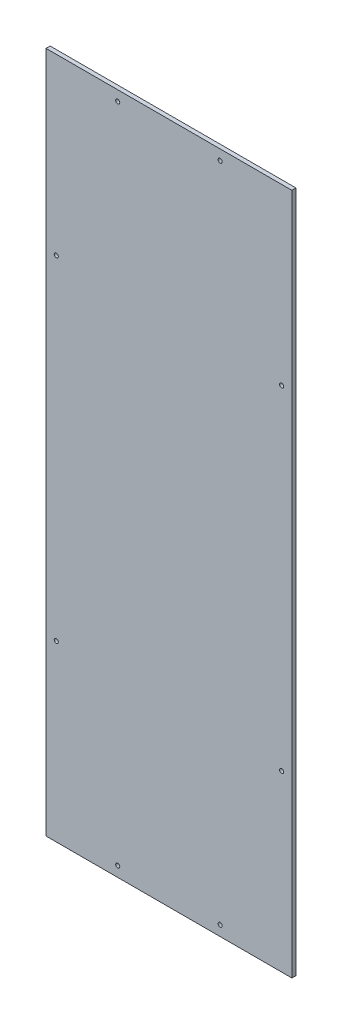
SolidWorks part; units mm, degrees
ref_plane "前视基准面" through (0, 0, 0) normal (0, 0, 1) x (1, 0, 0)
ref_plane "上视基准面" through (0, 0, 0) normal (0, 1, 0) x (1, 0, 0)
ref_plane "右视基准面" through (0, 0, 0) normal (1, 0, 0) x (0, 0, -1)
sketch "草图1" plane through (0, 0, 0) normal (0, 0, 1) x (1, 0, 0)
  line L1 (-120, -333) -> (120, -333)
  line L2 (-120, -333) -> (-120, 333)
  line L3 (-120, 333) -> (120, 333)
  line L4 (120, -333) -> (120, 333)
  line L5 (-120, -333) -> (120, 333) construction
  line L6 (-120, 333) -> (120, -333) construction
  point P0 (0, 0)
  dimension "D1" = 240
  dimension "D2" = 666
extrude "凸台-拉伸1" add sketch "草图1" along normal mid plane 4
hole_wizard "Ø4.0 (4) 直径孔1" positions "草图2" profile "草图3" hole size "Ø4.0" standard "GB" end condition through all
sketch "草图2" plane through (0, 0, -2) normal (0, 0, -1) x (-1, 0, 0)
  line L0 (-120, -333) -> (-120, 333) construction
  line L1 (-120, 333) -> (120, 333) construction
  line L2 (120, -333) -> (-120, -333) construction
  point P0 (-110, 163)
  point P2 (-110, -163)
  dimension "D1" = 10
  dimension "D2" = 170
  dimension "D3" = 170
  dimension "D4" = 10
sketch "草图3" plane through (110, 163, -2) normal (1, 0, 0) x (0, 1, 0)
  line L0 (0, 0) -> (0, 4)
  line L1 (0, 4) -> (2, 4)
  line L2 (2, 4) -> (2, 0)
  line L5 (2, 0) -> (0, 0)
  line L11 (0, -6.35) -> (0, 107.95) construction
  dimension "通孔孔直径" = 4
  dimension "通孔孔深度" = 4
hole_wizard "Ø4.0 (4) 直径孔2" positions "草图4" profile "草图5" hole size "Ø4.0" standard "GB" end condition through all
sketch "草图4" plane through (0, 0, -2) normal (0, 0, -1) x (-1, 0, 0)
  line L0 (-120, 333) -> (120, 333) construction
  line L1 (-120, -333) -> (-120, 333) construction
  line L2 (120, 333) -> (120, -333) construction
  point P0 (-50, 323)
  point P2 (50, 323)
  dimension "D1" = 10
  dimension "D2" = 70
  dimension "D3" = 70
  dimension "D4" = 10
sketch "草图5" plane through (50, 323, -2) normal (1, 0, 0) x (0, 1, 0)
  line L0 (0, 0) -> (0, 4)
  line L1 (0, 4) -> (2, 4)
  line L2 (2, 4) -> (2, 0)
  line L5 (2, 0) -> (0, 0)
  line L11 (0, -6.35) -> (0, 107.95) construction
  dimension "通孔孔直径" = 4
  dimension "通孔孔深度" = 4
mirror "镜向1" about plane through (0, 0, 0) normal (0, 1, 0) of "Ø4.0 (4) 直径孔2"
mirror "镜向2" about plane through (0, 0, 0) normal (1, 0, 0) of "Ø4.0 (4) 直径孔1"
